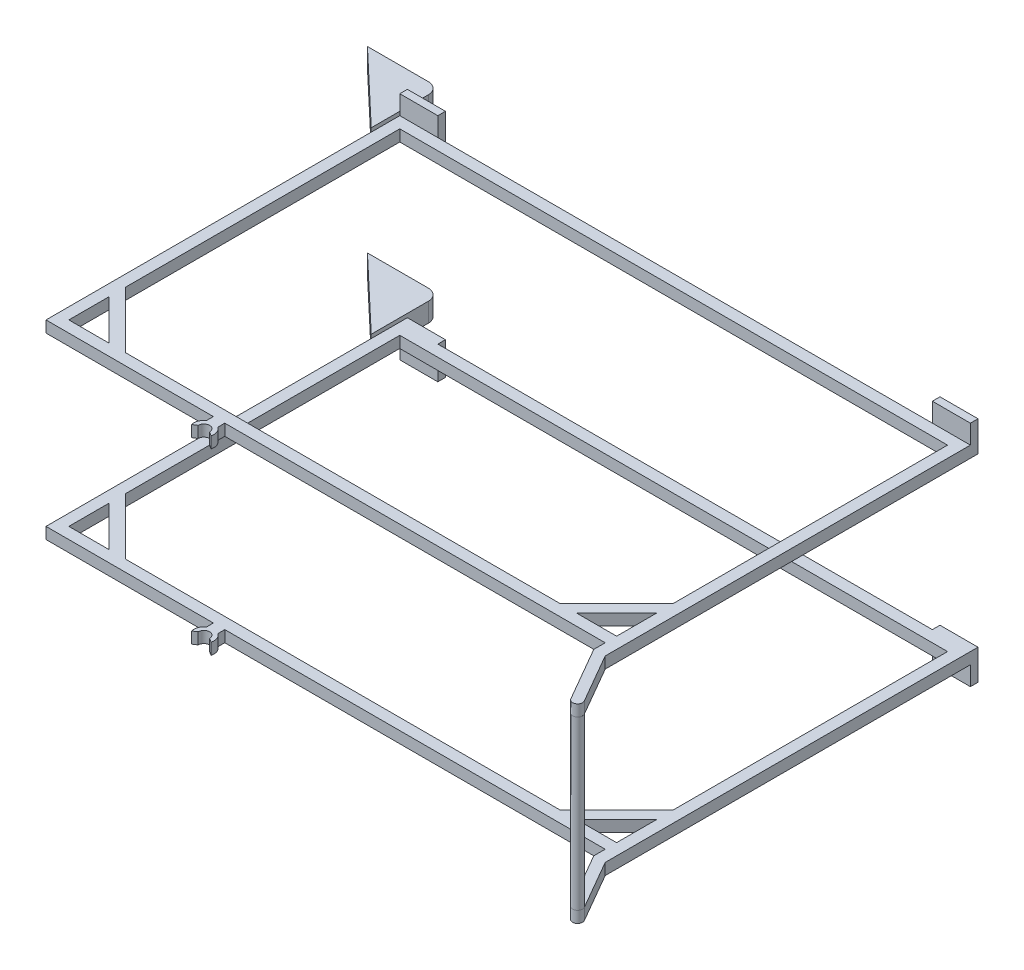
from build123d import *

# Parameters (mm, degrees)
SKETCH1_W            = 1500
SKETCH1_H            = 500
BOSS_EXTRUDE1_DEPTH  = 30
SKETCH2_W            = 30
SKETCH2_H            = 30
BOSS_EXTRUDE2_DEPTH  = 900
BOSS_EXTRUDE3_DEPTH  = 30
SKETCH4_W            = 30
SKETCH4_H            = 500
BOSS_EXTRUDE4_DEPTH  = 30
BOSS_EXTRUDE5_DEPTH  = 30
SKETCH6_R            = 12.990381057
BOSS_EXTRUDE6_DEPTH  = 500
BOSS_EXTRUDE7_DEPTH  = 30
BOSS_EXTRUDE8_DEPTH  = 300
FILLET1_R            = 30
SKETCH11_W           = 960
SKETCH11_H           = 500
BOSS_EXTRUDE9_DEPTH  = 30
SKETCH12_W           = 40
SKETCH12_H           = 220
CUT_EXTRUDE1_DEPTH   = 300
SKETCH13_W           = 1153.001247693
SKETCH13_H           = 440
CUT_EXTRUDE2_DEPTH   = 2083.426213795
BOSS_EXTRUDE11_DEPTH = 25
SKETCH16_W           = 100
SKETCH16_H           = 80
SKETCH16_H_2         = 85.940855112
BOSS_EXTRUDE12_DEPTH = 20


with BuildPart() as part:
    # Sketch1 → Boss-Extrude1 (new body)
    with BuildSketch(Plane.XY):
        with Locations((-750, -250)):
            Rectangle(SKETCH1_W, SKETCH1_H)
    extrude(amount=BOSS_EXTRUDE1_DEPTH)

    # Sketch2 → Boss-Extrude2 (add)
    with BuildSketch(Plane.XY.offset(30)):
        with Locations((-1485, -485)):
            Rectangle(SKETCH2_W, SKETCH2_H)
        with Locations((-1485, -15)):
            Rectangle(SKETCH2_W, SKETCH2_H)
        with Locations((-15, -15)):
            Rectangle(SKETCH2_W, SKETCH2_H)
        with Locations((-15, -485)):
            Rectangle(SKETCH2_W, SKETCH2_H)
    extrude(amount=BOSS_EXTRUDE2_DEPTH)

    # Sketch3 → Boss-Extrude3 (add)
    with BuildSketch(Plane.XZ.offset(500)):
        Polygon((-1500, 930), (0, 930), (0, 900), (-136.066017178, 900), (-30, 793.933982822), (-30, 751.507575951), (-178.492424049, 900), (-1321.507575951, 900), (-1470, 751.507575951), (-1470, 793.933982822), (-1363.933982822, 900), (-1500, 900), align=None)
    boss_extrude3 = extrude(amount=-BOSS_EXTRUDE3_DEPTH)

    # Mirror2: Boss-Extrude3 across plane
    add(boss_extrude3.mirror(Plane.ZX.offset(-250)))

    # Sketch4 → Boss-Extrude4 (add)
    with BuildSketch(Plane.XY.offset(930)):
        with Locations((-15, -250)):
            Rectangle(SKETCH4_W, SKETCH4_H)
    extrude(amount=BOSS_EXTRUDE4_DEPTH)

    # Sketch5 → Boss-Extrude5 (add)
    with BuildSketch(Plane.XZ.offset(500)):
        with BuildLine():
            Line((0, 960), (75, 1089.903810568))
            ThreePointArc((75, 1089.903810568), (70.155088258, 1107.492939386), (52.5, 1102.894191624))
            Line((52.5, 1102.894191624), (37.5, 1076.913429511))
            Line((37.5, 1076.913429511), (30.236347458, 1064.33241426))
            Line((30.236347458, 1064.33241426), (-30, 960))
            Line((-30, 960), (0, 960))
        make_face()
    boss_extrude5 = extrude(amount=-BOSS_EXTRUDE5_DEPTH)

    # Mirror3: Boss-Extrude5 across plane
    add(boss_extrude5.mirror(Plane.ZX.offset(-250)))

    # Sketch6 → Boss-Extrude6 (add)
    with BuildSketch(Plane.XZ.offset(500)):
        with Locations(Location((63.659263982, 1096.241841703, 0), (0, 0, 330))):
            Circle(SKETCH6_R)
    extrude(amount=-BOSS_EXTRUDE6_DEPTH)

    # Sketch8 → Boss-Extrude7 (add)
    with BuildSketch(Plane.XZ.offset(500)):
        with BuildLine():
            Line((-1060, 930), (-1030, 930))
            Line((-1030, 930), (-1030, 948.134875189))
            ThreePointArc((-1030, 948.134875189), (-1020.16081333, 960.721072878), (-1019.338342911, 976.675555288))
            Line((-1019.338342911, 976.675555288), (-1029.939297882, 970.038007257))
            ThreePointArc((-1029.939297882, 970.038007257), (-1045, 954.939249924), (-1060.060702118, 970.038007257))
            Line((-1060.060702118, 970.038007257), (-1070.661657089, 976.675555288))
            ThreePointArc((-1070.661657089, 976.675555288), (-1069.83918667, 960.721072878), (-1060, 948.134875189))
            Line((-1060, 948.134875189), (-1060, 930))
        make_face()
    boss_extrude7 = extrude(amount=-BOSS_EXTRUDE7_DEPTH)

    # Mirror4: Boss-Extrude7 across plane
    add(boss_extrude7.mirror(Plane.ZX.offset(-250)))

    # Sketch10 → Boss-Extrude8 (add)
    with BuildSketch(Plane.XZ.offset(500)):
        Polygon((-1500, 75), (-1500, -105), (-1690, -105), align=None)
    extrude(amount=-BOSS_EXTRUDE8_DEPTH)

    # Fillet1
    fillet1_edges = [part.edges().sort_by_distance(p)[0] for p in [
        (-1500, -350, -105),
    ]]
    fillet(fillet1_edges, radius=FILLET1_R)

    # Sketch11 → Boss-Extrude9 (add)
    with BuildSketch(Plane(origin=(0, 0, 0), x_dir=(0, 0, -1), z_dir=(1, 0, 0))):
        with Locations((-480, -250)):
            Rectangle(SKETCH11_W, SKETCH11_H)
    extrude(amount=-BOSS_EXTRUDE9_DEPTH)

    # Sketch12 → Cut-Extrude1 (cut)
    with BuildSketch(Plane(origin=(0, 0, 0), x_dir=(0, 0, -1), z_dir=(1, 0, 0))):
        with Locations((-70, -350)):
            Rectangle(SKETCH12_W, SKETCH12_H)
    extrude(amount=-CUT_EXTRUDE1_DEPTH, mode=Mode.SUBTRACT)

    # Sketch13 → Cut-Extrude2 (cut, through all)
    with BuildSketch(Plane(origin=(0, 0, 0), x_dir=(0, 0, -1), z_dir=(1, 0, 0))):
        with Locations((-383.499376154, -250)):
            Rectangle(SKETCH13_W, SKETCH13_H)
    extrude(amount=-CUT_EXTRUDE2_DEPTH, mode=Mode.SUBTRACT)

    # Sketch15 → Boss-Extrude11 (add, symmetric)
    with BuildSketch(Plane(origin=(0, -485, 0), x_dir=(-1, 0, 0), z_dir=(0, -1, 0))):
        with BuildLine():
            Line((1500, -75), (1500, 0))
            Line((1500, 0), (1500, 75))
            ThreePointArc((1500, 75), (1508.786796564, 96.213203436), (1530, 105))
            Line((1530, 105), (1690, 105))
            Line((1690, 105), (1500, -75))
        make_face()
    boss_extrude11 = extrude(amount=BOSS_EXTRUDE11_DEPTH, both=True)

    # Mirror5: Boss-Extrude11 across plane
    add(boss_extrude11.mirror(Plane.ZX.offset(-250)))

    # Sketch16 → Boss-Extrude12 (add)
    with BuildSketch(Plane(origin=(0, 0, 0), x_dir=(-1, 0, 0), z_dir=(0, 0, -1))):
        with Locations((1450, 10)):
            Rectangle(SKETCH16_W, SKETCH16_H)
        with Locations((1450, -512.970427556)):
            Rectangle(SKETCH16_W, SKETCH16_H_2)
        with Locations((50, -510)):
            Rectangle(SKETCH16_W, SKETCH16_H)
        with Locations((50, 10)):
            Rectangle(SKETCH16_W, SKETCH16_H)
    extrude(amount=BOSS_EXTRUDE12_DEPTH)


solid = part.part
